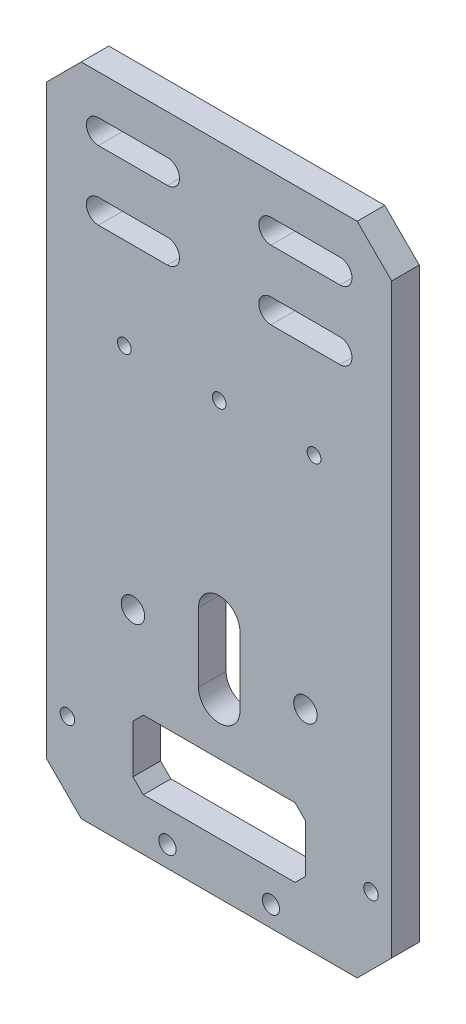
SolidWorks part; units mm, degrees
material "普通碳钢"
ref_plane "Front Plane" through (0, 0, 0) normal (0, 0, 1) x (1, 0, 0)
ref_plane "Top Plane" through (0, 0, 0) normal (0, 1, 0) x (1, 0, 0)
ref_plane "Right Plane" through (0, 0, 0) normal (1, 0, 0) x (0, 0, -1)
sketch "Sketch1" plane through (0, 0, 0) normal (0, 0, 1) x (1, 0, 0)
  line L0 (0, 180) -> (10, 190)
  line L1 (10, 0) -> (90, 0)
  line L2 (0, 10) -> (0, 180)
  line L3 (10, 190) -> (90, 190)
  line L4 (100, 10) -> (100, 180)
  line L5 (90, 190) -> (100, 180)
  line L6 (50, 190) -> (50, 40.0942) construction
  line L7 (25, 35) -> (75, 35)
  line L8 (25, 35) -> (25, 15)
  line L9 (25, 15) -> (75, 15)
  line L10 (75, 35) -> (75, 15)
  line L11 (25, 35) -> (75, 15) construction
  line L12 (25, 15) -> (75, 35) construction
  line L13 (35, 6) -> (65, 6) construction
  line L14 (10, 0) -> (0, 10)
  line L15 (90, 0) -> (100, 10)
  line L16 (50, 70) -> (50, 50) construction
  line L17 (56, 70) -> (56, 50)
  line L18 (44, 70) -> (44, 50)
  circle A0 centre (35, 6) radius 2.5
  circle A1 centre (65, 6) radius 2.5
  circle A2 centre (22.5, 125) radius 2
  circle A3 centre (50, 125) radius 2
  circle A4 centre (77.5, 125) radius 2
  arc A5 (56, 70) -> (44, 70) centre (50, 70) ccw
  arc A6 (44, 50) -> (56, 50) centre (50, 50) ccw
  point P0 (0, 0)
  point P1 (100, 190)
  point P2 (0, 190)
  point P3 (100, 0)
  point P13 (50, 25)
  point P20 (50, 6)
  point P33 (50, 60)
  dimension "D8" = 6
  dimension "D10" = 5
  dimension "D11" = 27.5
  dimension "D15" = 4
  dimension "D1" = 100
  dimension "D2" = 190
  dimension "D3" = 50
  dimension "D4" = 20
  dimension "D7" = 15
  dimension "D9" = 30
  dimension "D12" = 27.5
  dimension "D16" = 125
  dimension "D17" = 20
  dimension "D18" = 12
  dimension "D19" = 60
extrude "Boss-Extrude1" add sketch "Sketch1" along normal blind 8
cosmetic thread "Cosmetic Thread1" parameters "D2"=5
cosmetic thread "Cosmetic Thread2" parameters "D2"=5
cosmetic thread "Cosmetic Thread3" parameters "D2"=5
cosmetic thread "Cosmetic Thread4" parameters "D2"=6
cosmetic thread "Cosmetic Thread5" parameters "D2"=6
chamfer "Chamfer1" distance 3 angle 45 4 edges at (25, 35, 4) (75, 35, 4) (75, 15, 4) (25, 15, 4)
hole_wizard "Tap Drill for M8 Tap1" positions "3DSketch1" profile "Sketch2" hole size "M8" standard "GB"
sketch3d "3DSketch1"
  line L3 (50, 190, 8) -> (50, 0, 8) construction
  line L4 (90, 190, 8) -> (10, 190, 8) construction
  line L5 (10, 0, 8) -> (90, 0, 8) construction
  line L9 (44, 70, 8) -> (44, 50, 8) construction
  point P0 (25, 60, 8)
  point P2 (75, 60, 8)
  point P23 (44, 60, 8)
  dimension "D1" = 50
  dimension "D2" = 25
sketch "Sketch2" plane through (25, 60, 8) normal (1, 0, 0) x (0, -1, 0)
  line L0 (0, 0) -> (0, 17.0429)
  line L1 (0, 17.0429) -> (3.4, 15)
  line L2 (3.4, 15) -> (3.4, 0)
  line L5 (3.4, 0) -> (0, 0)
  line L10 (0, 17.0429) -> (-3.4, 15) construction
  line L11 (0, -6.35) -> (0, 107.95) construction
  dimension "孔直径" = 6.8
  dimension "孔深度" = 15
  dimension "导头角度" = 118
hole_wizard "Tap Drill for M5 Tap1" positions "3DSketch2" profile "Sketch4" hole size "M5" standard "GB"
sketch3d "3DSketch2"
  line L0 (100, 10, 0) -> (100, 180, 0) construction
  line L2 (10, 0, 8) -> (90, 0, 8) construction
  line L3 (50, 190, 0) -> (50, 0, 0) construction
  line L4 (90, 190, 0) -> (10, 190, 0) construction
  line L5 (10, 0, 0) -> (90, 0, 0) construction
  line L6 (0, 180, 0) -> (0, 10, 0) construction
  point P0 (94, 23.6854, 0)
  point P2 (6, 23.6854, 0)
  dimension "D1" = 6
  dimension "D2" = 6
  dimension "D3" = 25
sketch "Sketch4" plane through (94, 23.6854, 0) normal (1, 0, 0) x (0, 1, 0)
  line L0 (0, 0) -> (0, 16.2618)
  line L1 (0, 16.2618) -> (2.1, 15)
  line L2 (2.1, 15) -> (2.1, 0)
  line L5 (2.1, 0) -> (0, 0)
  line L10 (0, 16.2618) -> (-2.1, 15) construction
  line L11 (0, -6.35) -> (0, 107.95) construction
  dimension "孔直径" = 4.2
  dimension "孔深度" = 15
  dimension "导头角度" = 118
sketch "Sketch5" plane through (0, 0, 0) normal (0, 0, -1) x (-1, 0, 0)
  line L0 (-15, 175) -> (-35, 175) construction
  line L1 (-90, 190) -> (-10, 190) construction
  line L2 (-50, 190) -> (-50, 120.3363) construction
  line L3 (-85, 175) -> (-65, 175) construction
  line L4 (-85, 178.5) -> (-65, 178.5)
  line L5 (-85, 171.5) -> (-65, 171.5)
  line L6 (-15, 178.5) -> (-35, 178.5)
  line L7 (-15, 171.5) -> (-35, 171.5)
  arc A2 (-85, 178.5) -> (-85, 171.5) centre (-85, 175) ccw
  arc A3 (-65, 171.5) -> (-65, 178.5) centre (-65, 175) ccw
  arc A6 (-15, 178.5) -> (-15, 171.5) centre (-15, 175) cw
  arc A7 (-35, 171.5) -> (-35, 178.5) centre (-35, 175) cw
  point P6 (-75, 175)
  point P17 (-25, 175)
  dimension "D1" = 15
  dimension "D2" = 20
  dimension "D3" = 15
  dimension "D4" = 50
  dimension "D6" = 7
extrude "Cut-Extrude1" cut sketch "Sketch5" against normal blind 10
pattern_linear "LPattern1" count 2 spacing 20 along (0, -1, 0) of "Cut-Extrude1"
